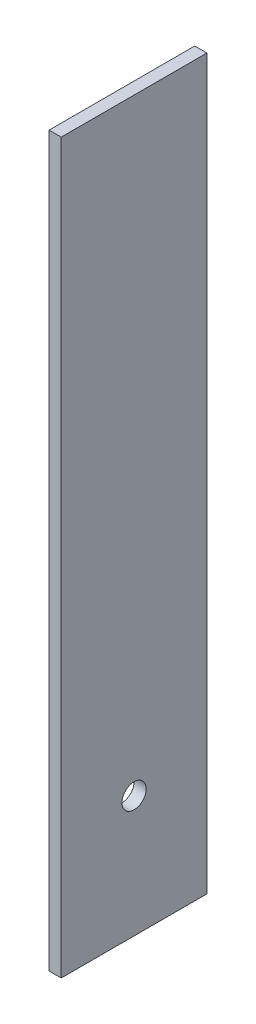
from build123d import *

# Parameters (mm, degrees)
SKETCH_1_W          = 5
SKETCH_1_H          = 300
EXTRUDE_1_DEPTH     = 60
SKETCH_2_R          = 5
CUT_EXTRUDE_1_DEPTH = 20


with BuildPart() as part:
    # 草图1 → 凸台-拉伸1 (new body)
    with BuildSketch(Plane.XY):
        Rectangle(SKETCH_1_W, SKETCH_1_H)
    extrude(amount=EXTRUDE_1_DEPTH)

    # 草图2 → 切除-拉伸1 (cut)
    with BuildSketch(Plane(origin=(2.5, 0, 0), x_dir=(0, 0, -1), z_dir=(1, 0, 0))):
        with Locations((-30, -100)):
            Circle(SKETCH_2_R)
    extrude(amount=-CUT_EXTRUDE_1_DEPTH, mode=Mode.SUBTRACT)


solid = part.part
